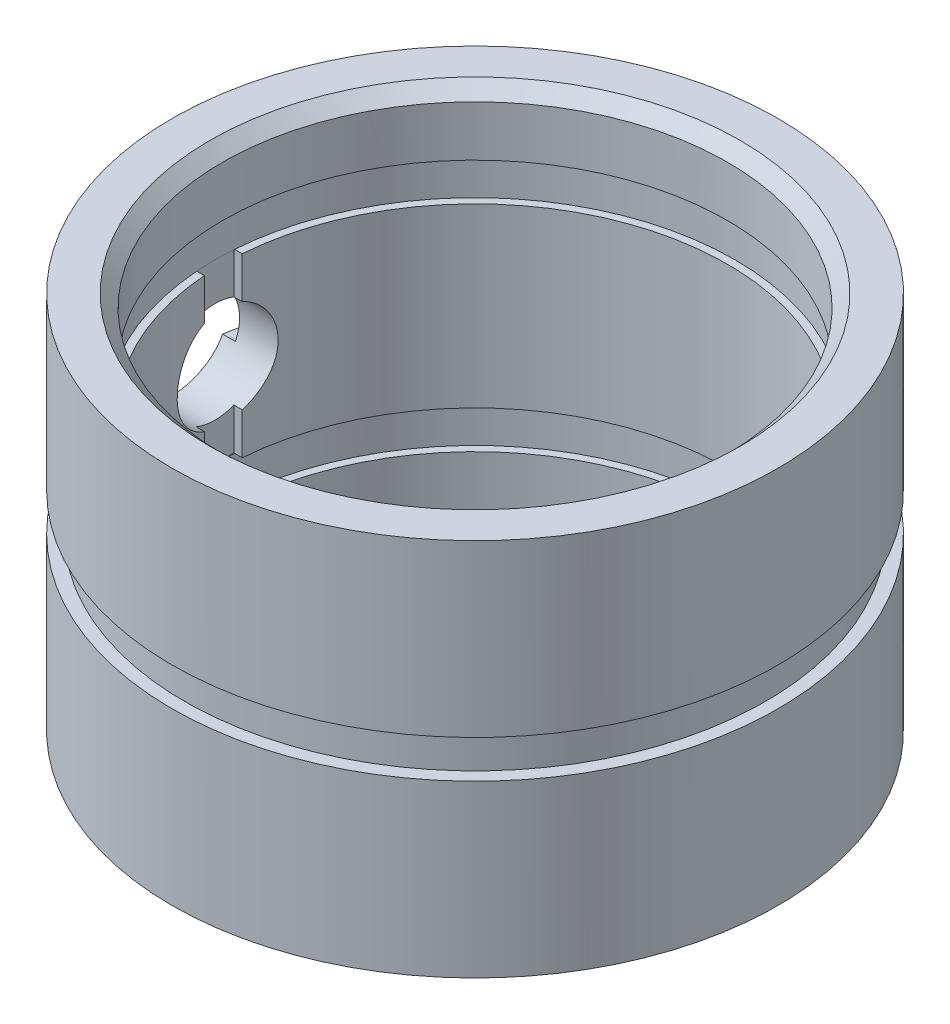
from build123d import *

# Parameters (mm, degrees)
SKETCH_1_R          = 24
SKETCH_1_R_2        = 20
EXTRUDE_1_DEPTH     = 15
SKETCH_2_W          = 20.6
SKETCH_2_H          = 3
SKETCH_2_W_2        = 4.5
SKETCH_5_W          = 3.1
SKETCH_5_H          = 3
CUT_EXTRUDE_1_DEPTH = 7
SKETCH_6_R          = 4
CUT_EXTRUDE_2_DEPTH = 38.107950631
CHAMFER_1_SIZE      = 1


with BuildPart() as part:
    # 草图1 → 凸台-拉伸1 (new, symmetric)
    with BuildSketch(Plane(origin=(0, 0, 0), x_dir=(1, 0, 0), z_dir=(0, 1, 0))):
        with Locations(Location((0, 0, 0), (0, 0, 270))):
            Circle(SKETCH_1_R)
        with Locations(Location((0, 0, 0), (0, 0, 270))):
            Circle(SKETCH_1_R_2, mode=Mode.SUBTRACT)
    extrude(amount=EXTRUDE_1_DEPTH, both=True)

    # 草图2 → 切除-旋转1 (revolve, cut)
    with BuildSketch(Plane.XY, mode=Mode.PRIVATE) as cut_revolve_1_sk:
        with Locations((10.3, 8.5)):
            Rectangle(SKETCH_2_W, SKETCH_2_H)
        with Locations((10.3, -8.5)):
            Rectangle(SKETCH_2_W, SKETCH_2_H)
        with Locations((25.25, 0)):
            Rectangle(SKETCH_2_W_2, SKETCH_2_H)
    revolve(cut_revolve_1_sk.sketch.rotate(Axis((0, 33.887302741, 0), (0, -1, 0)), 180), axis=Axis((0, 33.887302741, 0), (0, -1, 0)), mode=Mode.SUBTRACT)

    # 草图5 → 切除-拉伸1 (cut, symmetric)
    with BuildSketch(Plane(origin=(0, 0, 0), x_dir=(1, 0, 0), z_dir=(0, 1, 0))):
        with Locations((19.05, 0)):
            Rectangle(SKETCH_5_W, SKETCH_5_H)
        with Locations((-19.05, 0)):
            Rectangle(SKETCH_5_W, SKETCH_5_H)
    extrude(amount=CUT_EXTRUDE_1_DEPTH, both=True, mode=Mode.SUBTRACT)

    # 草图6 → 切除-拉伸2 (cut, through all)
    with BuildSketch(Plane(origin=(0, 0, 0), x_dir=(0, 0, -1), z_dir=(1, 0, 0))):
        with Locations(Location((0, 0, 0), (0, 0, 22.024312837))):
            Circle(SKETCH_6_R)
    extrude(amount=-CUT_EXTRUDE_2_DEPTH, mode=Mode.SUBTRACT)

    # 倒角1
    chamfer_1_edges = [part.edges().sort_by_distance(p)[0] for p in [
        (0, -15, -20),
        (0, 15, -20),
    ]]
    chamfer(chamfer_1_edges, length=CHAMFER_1_SIZE)


solid = part.part
